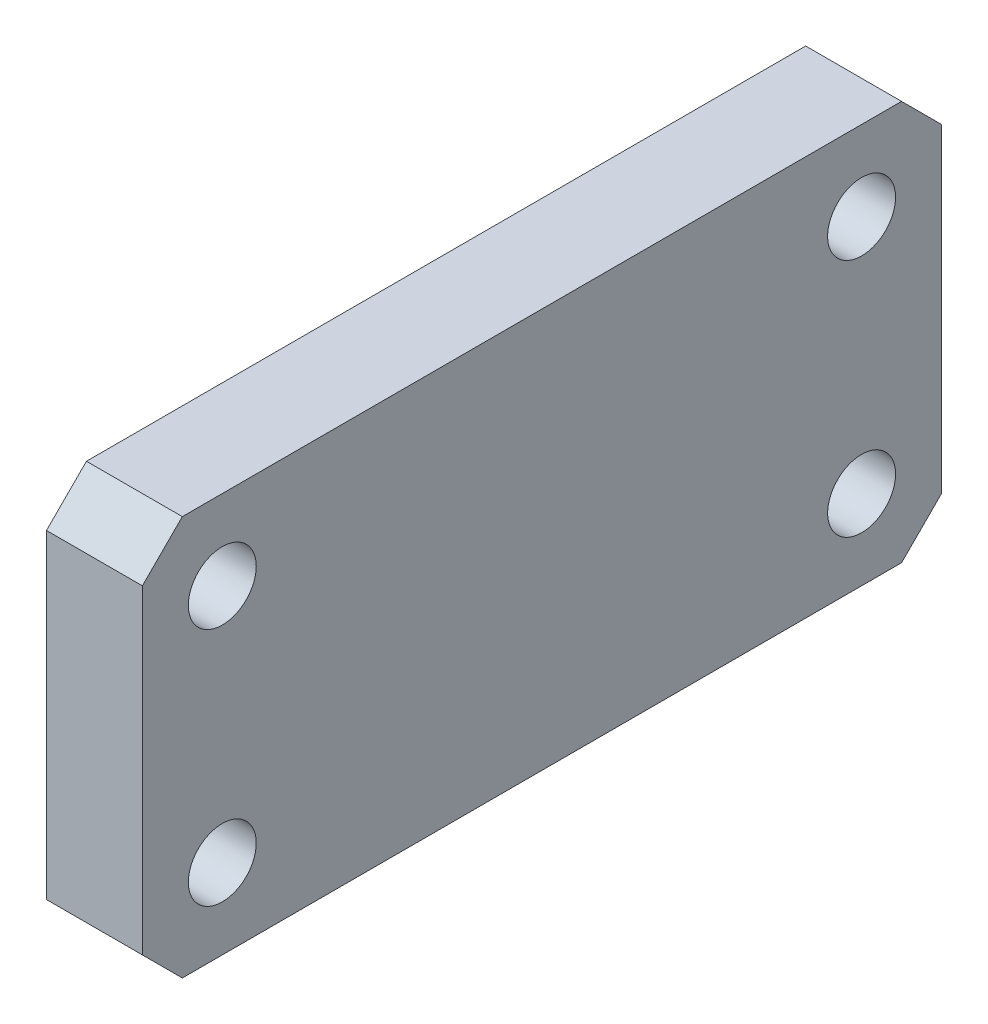
SolidWorks part; units mm, degrees
ref_plane "前视基准面" through (0, 0, 0) normal (0, 0, 1) x (1, 0, 0)
ref_plane "上视基准面" through (0, 0, 0) normal (0, 1, 0) x (1, 0, 0)
ref_plane "右视基准面" through (0, 0, 0) normal (1, 0, 0) x (0, 0, -1)
sketch "草图1" plane through (0, 0, 0) normal (1, 0, 0) x (0, 0, -1)
  line L1 (-50, 25) -> (50, 25)
  line L2 (-50, 25) -> (-50, -25)
  line L3 (-50, -25) -> (50, -25)
  line L4 (50, 25) -> (50, -25)
  line L5 (-50, 25) -> (50, -25) construction
  line L6 (-50, -25) -> (50, 25) construction
  point P0 (0, 0)
  dimension "D1" = 100
  dimension "D2" = 50
extrude "凸台-拉伸1" add sketch "草图1" along normal blind 12
hole_wizard "Ø8.5 (8.5) 直径孔1" positions "草图2" profile "草图3" hole size "Ø8.5" standard "GB" end condition through all
sketch "草图2" plane through (12, 0, 0) normal (1, 0, 0) x (0, 0, -1)
  line L0 (0, 62.2251) -> (0, 0) construction
  line L1 (0, 0) -> (70.822, 0) construction
  point P0 (-40, 15)
  point P2 (-40, -15)
  point P4 (40, 15)
  point P6 (40, -15)
  dimension "D1" = 80
  dimension "D2" = 30
sketch "草图3" plane through (12, 15, 40) normal (0, 1, 0) x (0, 0, -1)
  line L0 (0, 0) -> (0, 12)
  line L1 (0, 12) -> (4.25, 12)
  line L2 (4.25, 12) -> (4.25, 0)
  line L5 (4.25, 0) -> (0, 0)
  line L11 (0, -6.35) -> (0, 107.95) construction
  dimension "通孔孔直径" = 8.5
  dimension "通孔孔深度" = 12
chamfer "倒角1" distance 5 angle 45 4 edges at (6, 25, -50) (6, -25, -50) (6, 25, 50) (6, -25, 50)
